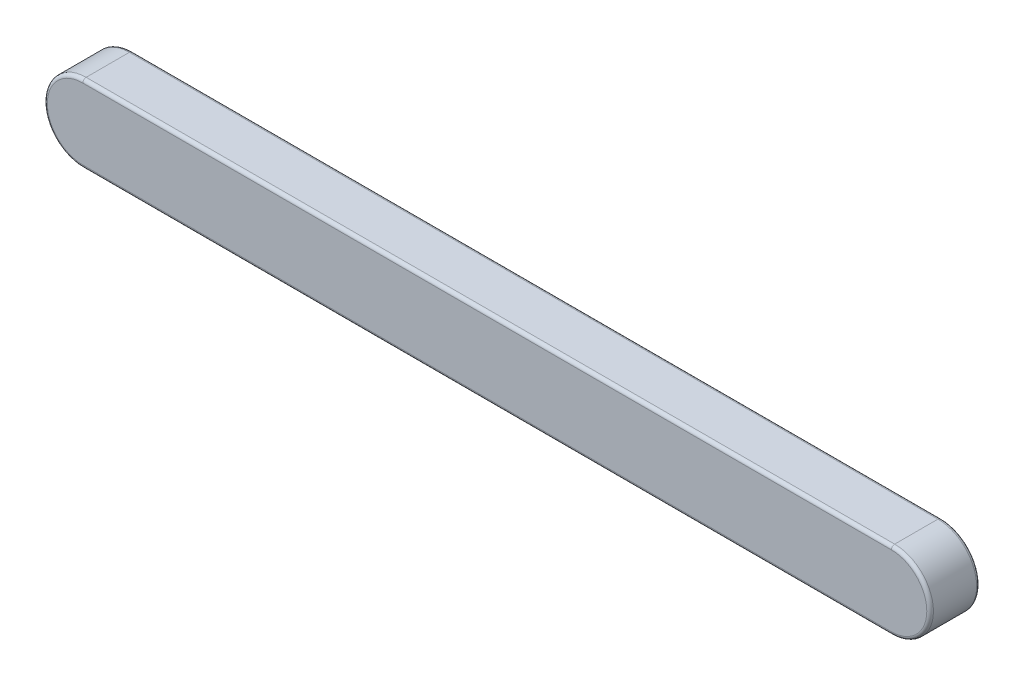
from build123d import *

# Parameters (mm, degrees)
BASE_EXTRUDE_DEPTH = 9
FILLET1_R          = 0.6


with BuildPart() as part:
    # Sketch1 → Base-Extrude (new body)
    with BuildSketch(Plane.XY):
        with BuildLine():
            Line((-73, 7), (73, 7))
            ThreePointArc((73, 7), (80, 0), (73, -7))
            Line((73, -7), (-73, -7))
            ThreePointArc((-73, -7), (-80, 0), (-73, 7))
        make_face()
    extrude(amount=BASE_EXTRUDE_DEPTH)

    # Fillet1
    fillet1_edges = [part.edges().sort_by_distance(p)[0] for p in [
        (80, 0, 9),
        (0, 7, 9),
        (-80, 0, 9),
        (0, 7, 0),
        (80, 0, 0),
        (0, -7, 0),
        (-80, 0, 0),
        (0, -7, 9),
    ]]
    fillet(fillet1_edges, radius=FILLET1_R)


solid = part.part
